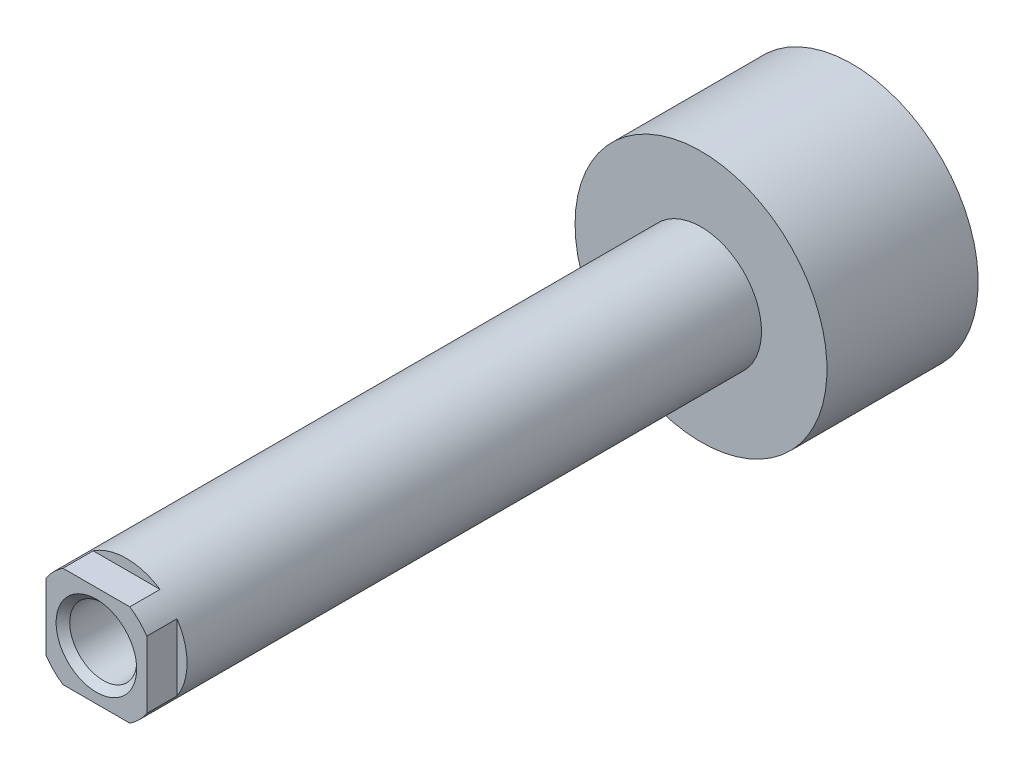
from build123d import *

# Parameters (mm, degrees)
SKETCH_2_R          = 10
SKETCH_2_W          = 10
SKETCH_2_H          = 10
CUT_EXTRUDE_1_DEPTH = 3


with BuildPart() as part:
    # 草图1 → 旋转1 (revolve)
    with BuildSketch(Plane(origin=(0, 0, 0), x_dir=(1, 0, 0), z_dir=(0, 1, 0)), mode=Mode.PRIVATE) as revolve_1_sk:
        Polygon((0, 54.5), (12.5, 54.5), (12.5, 39.5), (6, 39.5), (6, -20.5), (4, -20.5), (3.3235, -19.8235), (3.3235, -9.5), (0, -7.58117638), align=None)
    revolve(revolve_1_sk.sketch.rotate(Axis((0, 0, 20.5), (0, 0, -1)), 180), axis=Axis((0, 0, 20.5), (0, 0, -1)))

    # 草图2 → 切除-拉伸1 (cut)
    with BuildSketch(Plane.XY.offset(20.5)):
        Circle(SKETCH_2_R)
        Rectangle(SKETCH_2_W, SKETCH_2_H, mode=Mode.SUBTRACT)
    extrude(amount=-CUT_EXTRUDE_1_DEPTH, mode=Mode.SUBTRACT)


solid = part.part
